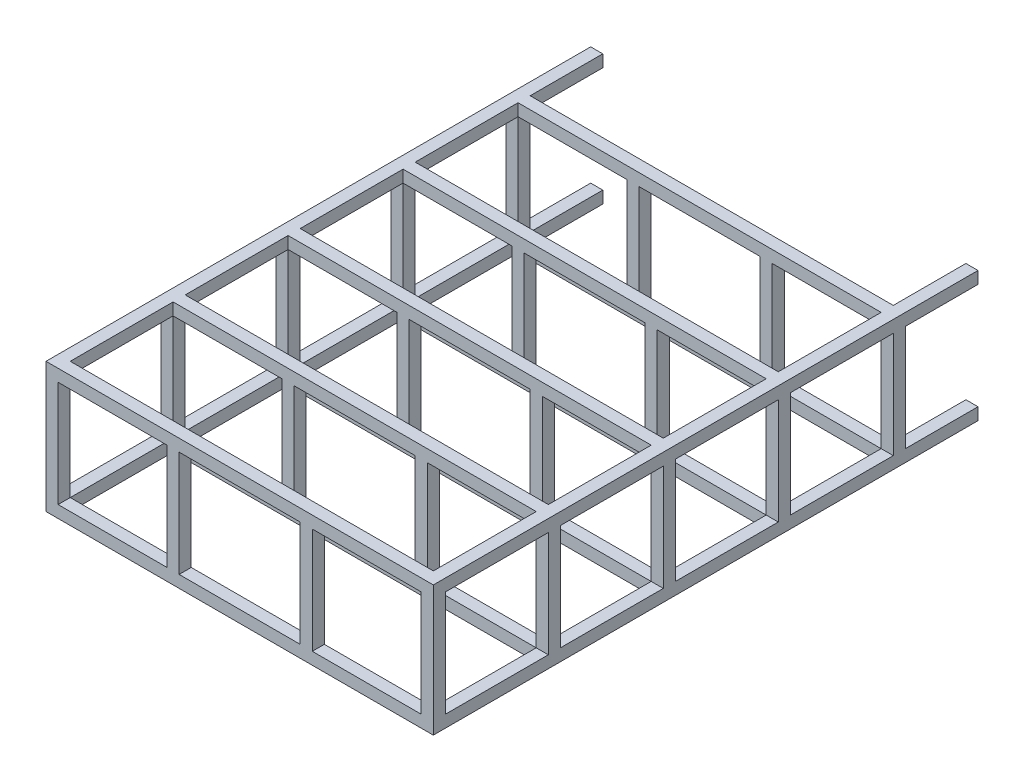
SolidWorks part; units mm, degrees
ref_plane "Front Plane" through (0, 0, 0) normal (0, 0, 1) x (1, 0, 0)
ref_plane "Top Plane" through (0, 0, 0) normal (0, 1, 0) x (1, 0, 0)
ref_plane "Right Plane" through (0, 0, 0) normal (1, 0, 0) x (0, 0, -1)
sketch "Sketch1" plane through (0, 0, 0) normal (0, 0, 1) x (1, 0, 0)
  line L0 (40, 390) -> (400, 390)
  line L1 (0, 0) -> (1280, 0)
  line L2 (0, 0) -> (0, 430)
  line L3 (0, 430) -> (1280, 430)
  line L4 (1280, 0) -> (1280, 430)
  line L5 (1240, 40) -> (1240, 390)
  line L6 (40, 40) -> (400, 40)
  line L7 (40, 40) -> (40, 390)
  line L8 (440, 390) -> (440, 40)
  line L9 (400, 390) -> (400, 40)
  line L10 (880, 40) -> (880, 390)
  line L11 (840, 390) -> (840, 40)
  line L12 (440, 390) -> (840, 390)
  line L13 (440, 40) -> (840, 40)
  line L14 (40, 390) -> (1240, 390) construction
  line L15 (880, 40) -> (1240, 40)
  line L16 (40, 40) -> (1240, 40) construction
  line L17 (880, 390) -> (1240, 390)
extrude "Boss-Extrude1" add sketch "Sketch1" along normal blind 40
sketch "Sketch2" plane through (0, 0, 40) normal (0, 0, 1) x (1, 0, 0)
  line L1 (0, 430) -> (40, 430)
  line L2 (0, 430) -> (0, 390)
  line L3 (0, 390) -> (40, 390)
  line L4 (40, 430) -> (40, 390)
  line L5 (40, 40) -> (0, 40)
  line L6 (40, 40) -> (40, 0)
  line L7 (40, 0) -> (0, 0)
  line L8 (0, 40) -> (0, 0)
  line L9 (1280, 0) -> (1240, 0)
  line L10 (1280, 0) -> (1280, 40)
  line L11 (1280, 40) -> (1240, 40)
  line L12 (1240, 0) -> (1240, 40)
  line L13 (1280, 430) -> (1240, 430)
  line L14 (1280, 430) -> (1280, 390)
  line L15 (1280, 390) -> (1240, 390)
  line L16 (1240, 430) -> (1240, 390)
extrude "Boss-Extrude2" add sketch "Sketch2" against normal blind 280 and the other way blind 1520
sketch "Sketch3" plane through (0, 0, 0) normal (0, -1, 0) x (1, 0, 0)
  line L0 (40, 1560) -> (40, 40) construction
  line L2 (0, 1560) -> (0, -240) construction
  line L3 (40, 380) -> (0, 380)
  line L4 (40, 380) -> (40, 420)
  line L5 (40, 420) -> (0, 420)
  line L6 (0, 380) -> (0, 420)
  line L7 (1240, 1560) -> (1240, 40) construction
  line L8 (1240, 380) -> (1280, 380)
  line L9 (1240, 380) -> (1240, 420)
  line L10 (1240, 420) -> (1280, 420)
  line L11 (1280, 380) -> (1280, 420)
  line L12 (1280, 1560) -> (1280, -240) construction
  line L14 (40, 760) -> (0, 760)
  line L15 (40, 760) -> (40, 800)
  line L16 (40, 800) -> (0, 800)
  line L17 (0, 760) -> (0, 800)
  line L18 (1240, 760) -> (1280, 760)
  line L19 (1240, 760) -> (1240, 800)
  line L20 (1240, 800) -> (1280, 800)
  line L21 (1280, 760) -> (1280, 800)
  line L22 (40, 1140) -> (0, 1140)
  line L23 (40, 1140) -> (40, 1180)
  line L24 (40, 1180) -> (0, 1180)
  line L25 (0, 1140) -> (0, 1180)
  line L26 (1240, 1140) -> (1280, 1140)
  line L27 (1240, 1140) -> (1240, 1180)
  line L28 (1240, 1180) -> (1280, 1180)
  line L29 (1280, 1140) -> (1280, 1180)
  line L30 (40, 1520) -> (0, 1520)
  line L31 (40, 1520) -> (40, 1560)
  line L32 (40, 1560) -> (0, 1560)
  line L33 (0, 1520) -> (0, 1560)
  line L34 (1240, 1520) -> (1280, 1520)
  line L35 (1240, 1520) -> (1240, 1560)
  line L36 (1240, 1560) -> (1280, 1560)
  line L37 (1280, 1520) -> (1280, 1560)
  point P0 (40, 380)
  point P19 (40, 760)
  point P28 (40, 1140)
  point P37 (40, 1520)
extrude "Boss-Extrude3" add sketch "Sketch3" against normal blind 411
sketch "Sketch4" plane through (0, 0, 0) normal (-1, 0, 0) x (0, 0, 1)
  line L0 (1560, 430) -> (-240, 430) construction
  line L1 (0, 390) -> (40, 390)
  line L2 (0, 390) -> (0, 430)
  line L3 (0, 430) -> (40, 430)
  line L4 (40, 390) -> (40, 430)
  line L5 (1560, 0) -> (-240, 0) construction
  line L6 (0, 40) -> (40, 40)
  line L7 (0, 40) -> (0, 0)
  line L8 (0, 0) -> (40, 0)
  line L9 (40, 40) -> (40, 0)
  line L11 (380, 40) -> (420, 40)
  line L12 (380, 40) -> (380, 0)
  line L13 (380, 0) -> (420, 0)
  line L14 (420, 40) -> (420, 0)
  line L15 (380, 390) -> (420, 390)
  line L16 (380, 390) -> (380, 430)
  line L17 (380, 430) -> (420, 430)
  line L18 (420, 390) -> (420, 430)
  line L19 (760, 390) -> (800, 390)
  line L20 (760, 390) -> (760, 430)
  line L21 (760, 430) -> (800, 430)
  line L22 (800, 390) -> (800, 430)
  line L23 (760, 40) -> (800, 40)
  line L24 (760, 40) -> (760, 0)
  line L25 (760, 0) -> (800, 0)
  line L26 (800, 40) -> (800, 0)
  line L27 (1140, 40) -> (1180, 40)
  line L28 (1140, 40) -> (1140, 0)
  line L29 (1140, 0) -> (1180, 0)
  line L30 (1180, 40) -> (1180, 0)
  line L31 (1140, 390) -> (1180, 390)
  line L32 (1140, 390) -> (1140, 430)
  line L33 (1140, 430) -> (1180, 430)
  line L34 (1180, 390) -> (1180, 430)
  line L35 (1520, 390) -> (1560, 390)
  line L36 (1520, 390) -> (1520, 430)
  line L37 (1520, 430) -> (1560, 430)
  line L38 (1560, 390) -> (1560, 430)
  line L39 (1520, 40) -> (1560, 40)
  line L40 (1520, 40) -> (1520, 0)
  line L41 (1520, 0) -> (1560, 0)
  line L42 (1560, 40) -> (1560, 0)
extrude "Boss-Extrude4" add sketch "Sketch4" against normal up to vertex (1240 mm away)
sketch "Sketch5" plane through (0, 0, 0) normal (0, -1, 0) x (1, 0, 0)
  line L0 (40, 40) -> (1240, 40) construction
  line L1 (440, 40) -> (400, 40)
  line L2 (440, 40) -> (440, 0)
  line L3 (440, 0) -> (400, 0)
  line L4 (400, 40) -> (400, 0)
  line L5 (40, 0) -> (1240, 0) construction
  line L6 (40, 380) -> (40, 40) construction
  line L8 (840, 40) -> (840, 0)
  line L9 (1240, 380) -> (1240, 40) construction
  line L10 (840, 40) -> (880, 40)
  line L12 (880, 40) -> (880, 0)
  line L13 (880, 0) -> (840, 0)
  line L14 (1240, 380) -> (40, 380) construction
  line L15 (400, 380) -> (440, 380)
  line L16 (400, 380) -> (400, 420)
  line L17 (400, 420) -> (440, 420)
  line L18 (440, 380) -> (440, 420)
  line L19 (1240, 420) -> (40, 420) construction
  line L20 (1240, 760) -> (40, 760) construction
  line L21 (840, 380) -> (880, 380)
  line L22 (840, 380) -> (840, 420)
  line L23 (840, 420) -> (880, 420)
  line L24 (880, 380) -> (880, 420)
  line L25 (400, 760) -> (440, 760)
  line L26 (400, 760) -> (400, 800)
  line L27 (400, 800) -> (440, 800)
  line L28 (440, 760) -> (440, 800)
  line L29 (1240, 800) -> (40, 800) construction
  line L30 (1240, 1140) -> (40, 1140) construction
  line L31 (840, 760) -> (880, 760)
  line L32 (840, 760) -> (840, 800)
  line L33 (840, 800) -> (880, 800)
  line L34 (880, 760) -> (880, 800)
  line L35 (400, 1140) -> (440, 1140)
  line L36 (400, 1140) -> (400, 1180)
  line L37 (400, 1180) -> (440, 1180)
  line L38 (440, 1140) -> (440, 1180)
  line L39 (1240, 1180) -> (40, 1180) construction
  line L40 (1240, 1520) -> (40, 1520) construction
  line L41 (840, 1140) -> (880, 1140)
  line L42 (840, 1140) -> (840, 1180)
  line L43 (840, 1180) -> (880, 1180)
  line L44 (880, 1140) -> (880, 1180)
  line L45 (880, 1520) -> (840, 1520)
  line L46 (880, 1520) -> (880, 1560)
  line L47 (880, 1560) -> (840, 1560)
  line L48 (840, 1520) -> (840, 1560)
  line L49 (1280, 1560) -> (0, 1560) construction
  line L51 (400, 1560) -> (440, 1560)
  line L52 (400, 1560) -> (400, 1520)
  line L53 (400, 1520) -> (440, 1520)
  line L54 (440, 1560) -> (440, 1520)
  dimension "D1" = 400
  dimension "D2" = 40
  dimension "D3" = 400
extrude "Boss-Extrude5" add sketch "Sketch5" against normal up to vertex (390 mm away)
